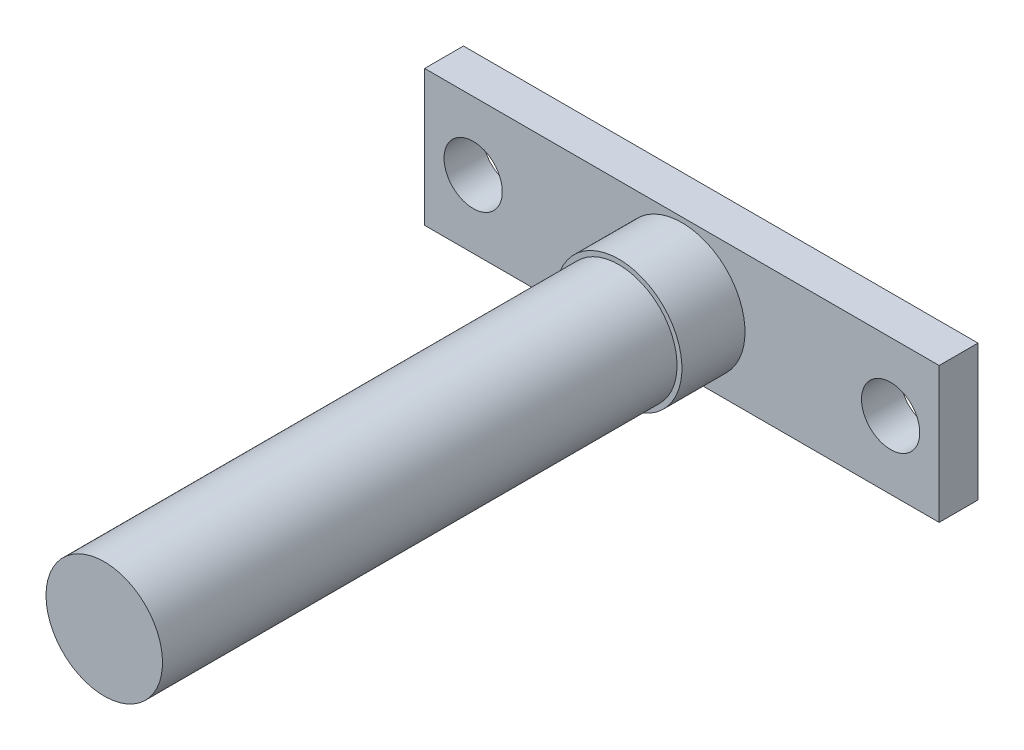
SolidWorks part; units mm, degrees
ref_plane "前视基准面" through (0, 0, 0) normal (0, 0, 1) x (1, 0, 0)
ref_plane "上视基准面" through (0, 0, 0) normal (0, 1, 0) x (1, 0, 0)
ref_plane "右视基准面" through (0, 0, 0) normal (1, 0, 0) x (0, 0, -1)
sketch "草图1" plane through (0, 0, 0) normal (0, 0, 1) x (1, 0, 0)
  circle A0 centre (0, 0) radius 6
  dimension "D1" = 12
extrude "凸台-拉伸1" add sketch "草图1" along normal blind 59.5
sketch "草图2" plane through (0, 0, 0) normal (0, 0, -1) x (-1, 0, 0)
  line L1 (-26.5, -7) -> (26.5, -7)
  line L2 (-26.5, -7) -> (-26.5, 7)
  line L3 (-26.5, 7) -> (26.5, 7)
  line L4 (26.5, -7) -> (26.5, 7)
  line L5 (-26.5, -7) -> (26.5, 7) construction
  line L6 (-26.5, 7) -> (26.5, -7) construction
  circle A0 centre (-21.5, 0) radius 3
  circle A1 centre (21.5, 0) radius 3
  point P0 (0, 0)
  dimension "D4" = 6
  dimension "D1" = 53
  dimension "D2" = 14
  dimension "D3" = 5
  dimension "D5" = 5
extrude "凸台-拉伸2" add sketch "草图2" along normal blind 4
sketch "草图3" plane through (0, 0, 0) normal (0, 0, 1) x (1, 0, 0)
  circle A0 centre (0, 0) radius 6.5
  dimension "D1" = 13
extrude "凸台-拉伸3" add sketch "草图3" along normal blind 6.5
